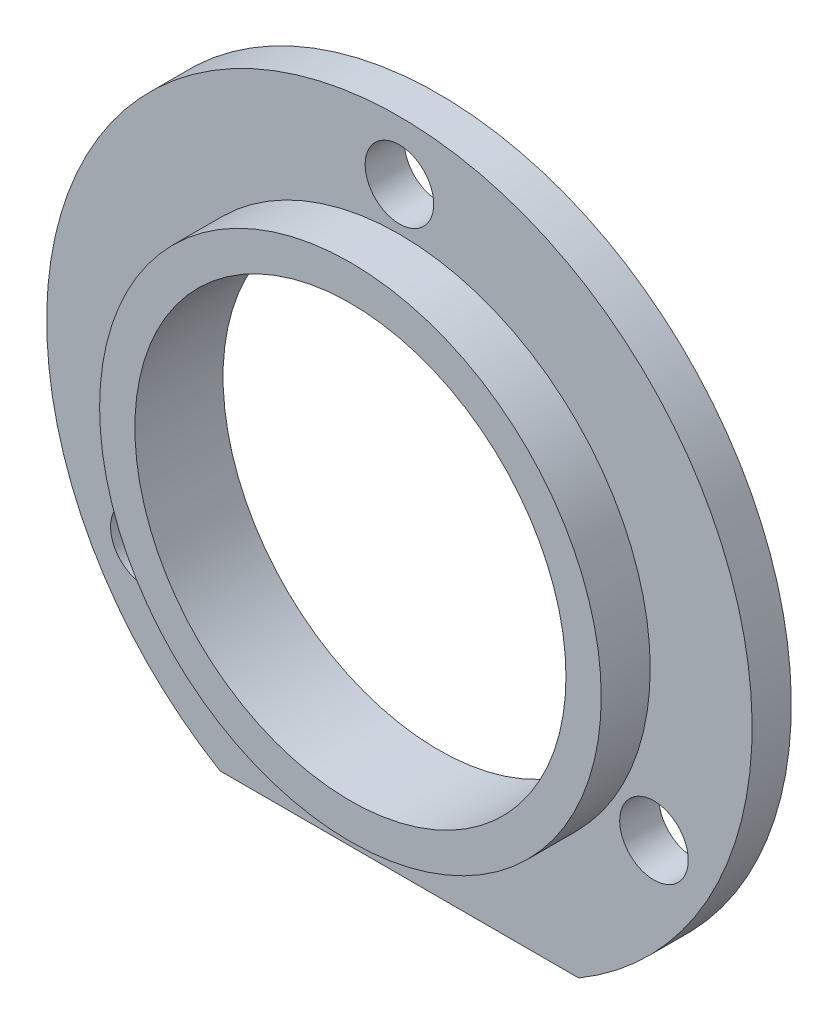
from build123d import *

# Parameters (mm, degrees)
SKETCH_1_R          = 18
SKETCH_1_R_2        = 11
EXTRUDE_1_DEPTH     = 4.5
SKETCH_2_OUTSIDE_W  = 48.222
SKETCH_2_OUTSIDE_H  = 48.222
SKETCH_2_OUTSIDE_R  = 12.8
CUT_EXTRUDE_1_DEPTH = 2.5
SKETCH_3_W          = 45.784626658
SKETCH_3_H          = 5.372844692
CUT_EXTRUDE_2_DEPTH = 26.578311125
SKETCH_4_R          = 1.75
CUT_EXTRUDE_3_DEPTH = 26.850531909


with BuildPart() as part:
    # 草图1 → 凸台-拉伸1 (new body)
    with BuildSketch(Plane.XY):
        Circle(SKETCH_1_R)
        Circle(SKETCH_1_R_2, mode=Mode.SUBTRACT)
    extrude(amount=EXTRUDE_1_DEPTH)

    # 草图2 outside → 切除-拉伸1 (cut)
    with BuildSketch(Plane.XY.offset(4.5)):
        Rectangle(SKETCH_2_OUTSIDE_W, SKETCH_2_OUTSIDE_H)
        Circle(SKETCH_2_OUTSIDE_R, mode=Mode.SUBTRACT)
    extrude(amount=-CUT_EXTRUDE_1_DEPTH, mode=Mode.SUBTRACT)

    # 草图3 → 切除-拉伸2 (cut, through all)
    with BuildSketch(Plane.XY.offset(2)):
        with Locations((-1.895541868, -18.186422346)):
            Rectangle(SKETCH_3_W, SKETCH_3_H)
    extrude(amount=-CUT_EXTRUDE_2_DEPTH, mode=Mode.SUBTRACT)

    # 草图4 → 切除-拉伸3 (cut, through all)
    with BuildSketch(Plane(origin=(0, 0, 0), x_dir=(-1, 0, 0), z_dir=(0, 0, -1))):
        with Locations((0, 15)):
            Circle(SKETCH_4_R)
        with Locations((-12.990381057, -7.5)):
            Circle(SKETCH_4_R)
        with Locations((12.990381057, -7.5)):
            Circle(SKETCH_4_R)
    extrude(amount=-CUT_EXTRUDE_3_DEPTH, mode=Mode.SUBTRACT)


solid = part.part
